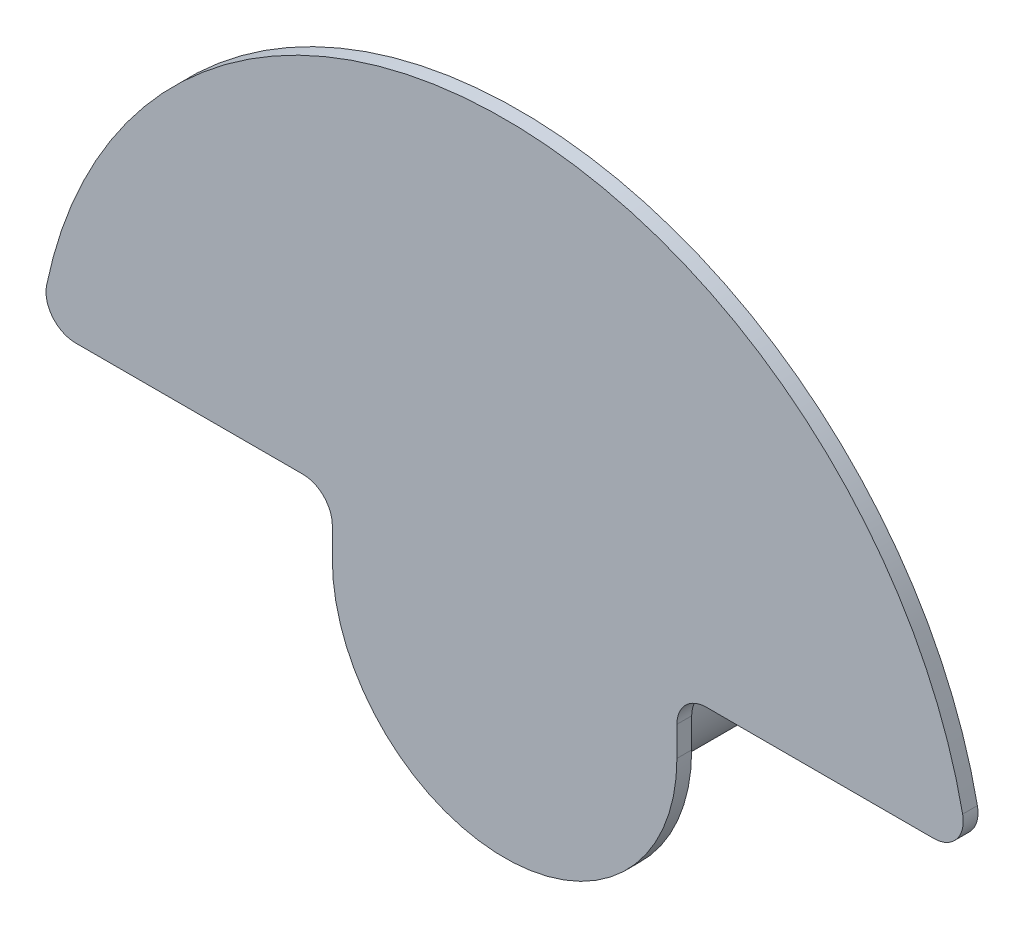
SolidWorks part; units mm, degrees
material "1023 碳钢板 (SS)"
ref_plane "前视基准面" through (0, 0, 0) normal (0, 0, 1) x (1, 0, 0)
ref_plane "上视基准面" through (0, 0, 0) normal (0, 1, 0) x (1, 0, 0)
ref_plane "右视基准面" through (0, 0, 0) normal (1, 0, 0) x (0, 0, -1)
ref_plane "基准面4" through (0, 0, 0.75) normal (0, 0, 1) x (1, 0, 0)
sketch "草图1" plane through (0, 0, 0.75) normal (0, 0, 1) x (1, 0, 0)
  line L0 (17.5, 6) -> (47.1195, 6)
  line L1 (-47.1195, 6) -> (-17.5, 6)
  line L2 (-17.5, 6) -> (-17.5, 0)
  line L3 (17.5, 0) -> (17.5, 6)
  arc A0 (47.1195, 6) -> (-47.1195, 6) centre (0, 0) ccw
  arc A1 (-17.5, 0) -> (17.5, 0) centre (0, 0) ccw
extrude "凸台-拉伸1" add sketch "草图1" against normal blind 1.5
sketch "草图2" plane through (0, 0, 0) normal (0, 1, 0) x (1, 0, 0)
  line L0 (12.5, 14.25) -> (0, 14.25)
  line L1 (0, 14.25) -> (0, 0.75)
  line L2 (0, 0.75) -> (12.5, 0.75)
  line L3 (12.5, 0.75) -> (12.5, 14.25)
  line L4 (0, 14.25) -> (0, 0.75) construction
revolve "旋转1" add sketch "草图2" angle 360 about L4
hole_wizard "Ø12.0 (12) 直径孔1" positions "草图4" profile "草图3" hole size "Ø12.0" standard "ANSI Metric"
sketch "草图4" plane through (0, 0, -14.25) normal (0, 0, -1) x (-1, 0, 0)
  point P0 (0, 0)
sketch "草图3" plane through (0, 0, -14.25) normal (1, 0, 0) x (0, 1, 0)
  line L0 (0, 0) -> (0, 13.5)
  line L1 (0, 13.5) -> (6, 13.5)
  line L2 (6, 13.5) -> (6, 0)
  line L5 (6, 0) -> (0, 0)
  line L10 (0, 13.5) -> (-6, 13.5) construction
  line L11 (0, -6.35) -> (0, 107.95) construction
  dimension "孔直径" = 12
  dimension "孔深度" = 13.5
  dimension "导头角度" = 180
ref_plane "基准面5" through (0, -5.7687, 0) normal (0, 1, 0) x (1, 0, 0)
hole_wizard "Ø3.3 (3.3) 直径孔1" positions "草图6" profile "草图5" hole size "Ø3.3" standard "ANSI Metric"
sketch "草图6" plane through (0, -5.7687, 0) normal (0, 1, 0) x (1, 0, 0)
  point P0 (0, 9.25)
sketch "草图5" plane through (0, -5.7687, -9.25) normal (1, 0, 0) x (0, 0, 1)
  line L0 (0, 0) -> (0, 11.7313)
  line L1 (0, 11.7313) -> (1.65, 11.7313)
  line L2 (1.65, 11.7313) -> (1.65, 0)
  line L5 (1.65, 0) -> (0, 0)
  line L11 (0, -6.35) -> (0, 107.95) construction
  dimension "通孔孔直径" = 3.3
  dimension "通孔孔深度" = 11.7313
ref_plane "基准面6" through (0, 5.7687, 0) normal (0, -1, 0) x (-1, 0, 0)
hole_wizard "Ø3.3 (3.3) 直径孔2" positions "草图8" profile "草图7" hole size "Ø3.3" standard "ANSI Metric"
sketch "草图8" plane through (0, 5.7687, 0) normal (0, -1, 0) x (-1, 0, 0)
  point P0 (0, 9.25)
sketch "草图7" plane through (0, 5.7687, -9.25) normal (1, 0, 0) x (0, 0, -1)
  line L0 (0, 0) -> (0, 41.7313)
  line L1 (0, 41.7313) -> (1.65, 41.7313)
  line L2 (1.65, 41.7313) -> (1.65, 0)
  line L5 (1.65, 0) -> (0, 0)
  line L11 (0, -6.35) -> (0, 107.95) construction
  dimension "通孔孔直径" = 3.3
  dimension "通孔孔深度" = 41.7313
fillet "圆角1" radius 3 4 edges at (-17.5, 6, 0) (-47.1195, 6, 0) (47.1195, 6, 0) (17.5, 6, 0)
